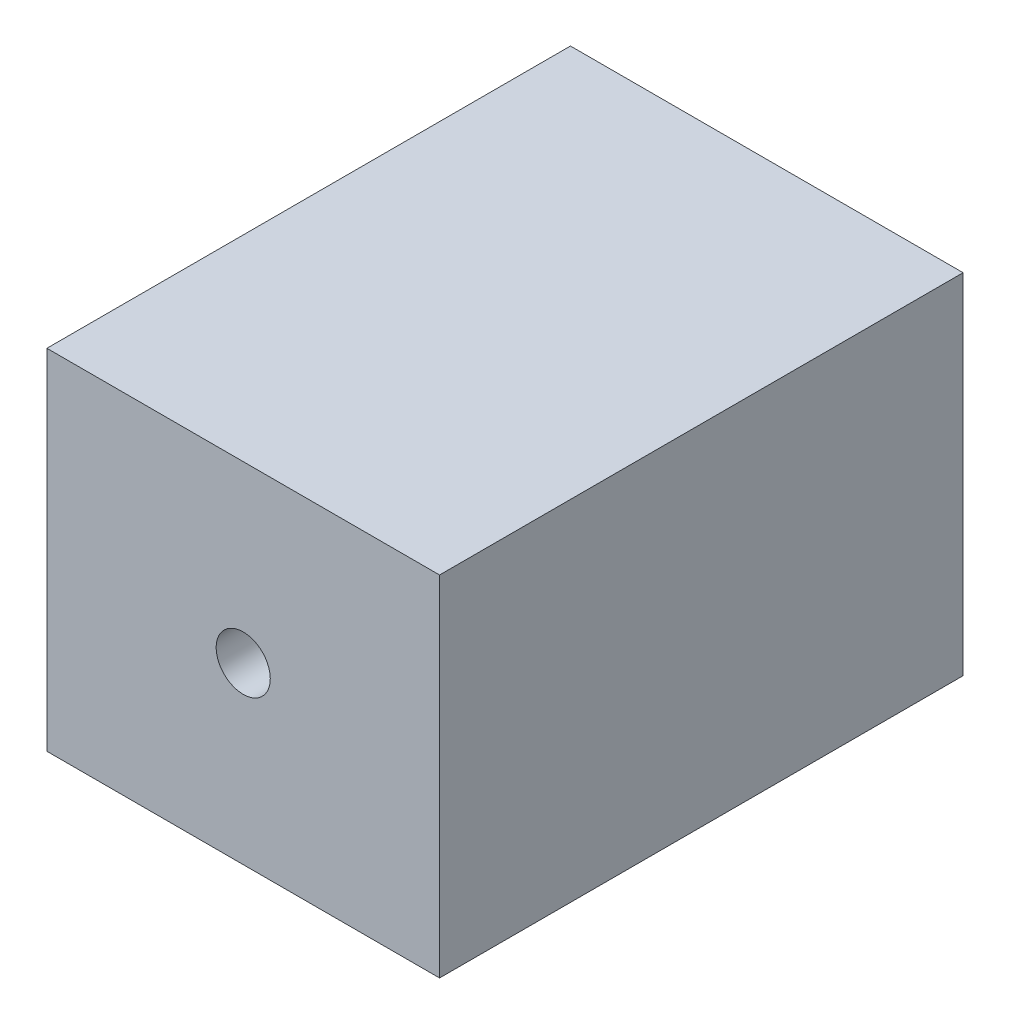
from build123d import *

# Parameters (mm, degrees)
SKETCH_1_W          = 90
SKETCH_1_H          = 80
EXTRUDE_1_DEPTH     = 60
SKETCH_2_R          = 6.2
CUT_EXTRUDE_1_DEPTH = 80


with BuildPart() as part:
    # 草图1 → 凸台-拉伸1 (new, symmetric)
    with BuildSketch(Plane.XY):
        Rectangle(SKETCH_1_W, SKETCH_1_H)
    extrude(amount=EXTRUDE_1_DEPTH, both=True)

    # 草图2 → 切除-拉伸1 (cut, symmetric)
    with BuildSketch(Plane.XY):
        Circle(SKETCH_2_R)
    extrude(amount=CUT_EXTRUDE_1_DEPTH, both=True, mode=Mode.SUBTRACT)


solid = part.part
